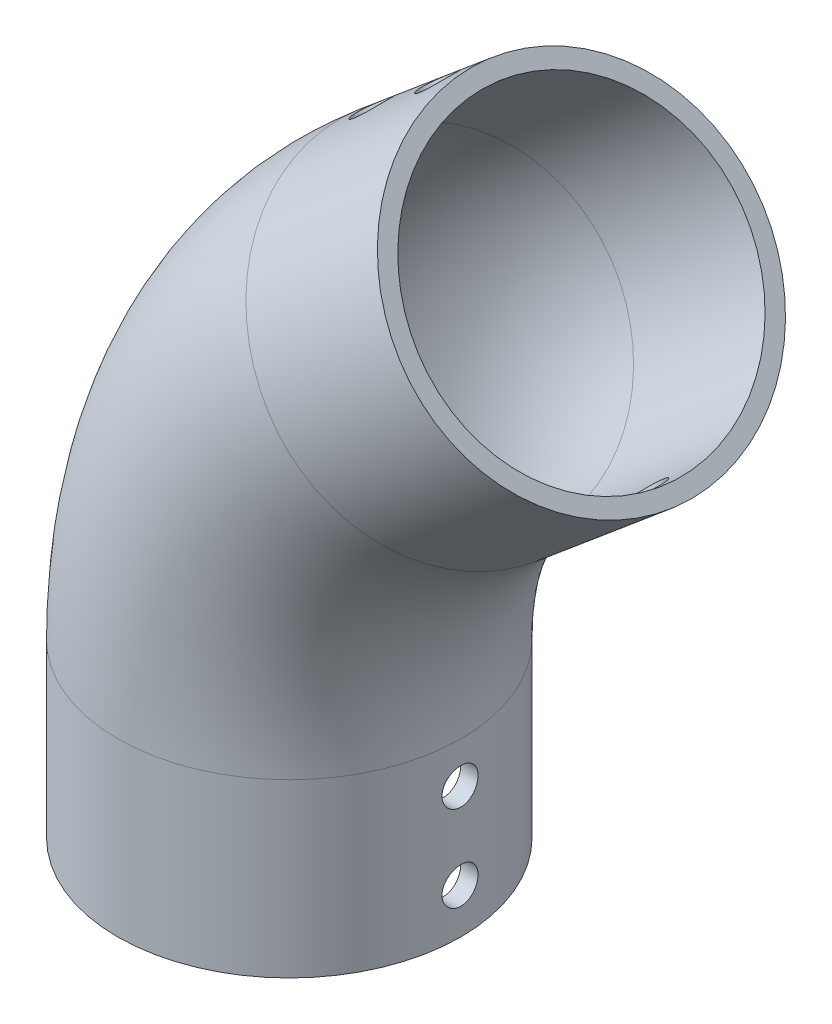
from build123d import *

# Parameters (mm, degrees)
SKETCH_3_R          = 50
SKETCH_3_R_2        = 45
SKETCH_4_R          = 5.25
CUT_EXTRUDE_1_DEPTH = 55


with BuildPart() as part:
    # 扫描2: sweep along a path in 草图1
    with BuildLine(Plane.XY) as sweep_2_path:
        Line((0, 0), (0, 50))
        ThreePointArc((0, 50), (12.273679898, 105.362992288), (46.794823131, 150.351822049))
        Line((46.794823131, 150.351822049), (85.097045287, 182.491202533))
    # 草图3 → 扫描2 (sweep)
    with BuildSketch(Plane(origin=(0, 0, 0), x_dir=(1, 0, 0), z_dir=(0, 1, 0))):
        Circle(SKETCH_3_R)
        Circle(SKETCH_3_R_2, mode=Mode.SUBTRACT)
    sweep(path=sweep_2_path.line)

    # 草图4 → 切除-拉伸1 (cut, symmetric)
    with BuildSketch(Plane(origin=(0, 0, 0), x_dir=(0, 0, -1), z_dir=(1, 0, 0))):
        with Locations((0, 13)):
            Circle(SKETCH_4_R)
        with Locations((0, 38)):
            Circle(SKETCH_4_R)
    cut_extrude_1 = extrude(amount=CUT_EXTRUDE_1_DEPTH, both=True, mode=Mode.SUBTRACT)

    # 镜向1: 切除-拉伸1 across plane
    add(cut_extrude_1.mirror(Plane(origin=(42.548522644, 91.245601266, 0), x_dir=(0, 0, 1), z_dir=(0.42261826174070016, 0.9063077870366497, 0))), mode=Mode.SUBTRACT)


solid = part.part
